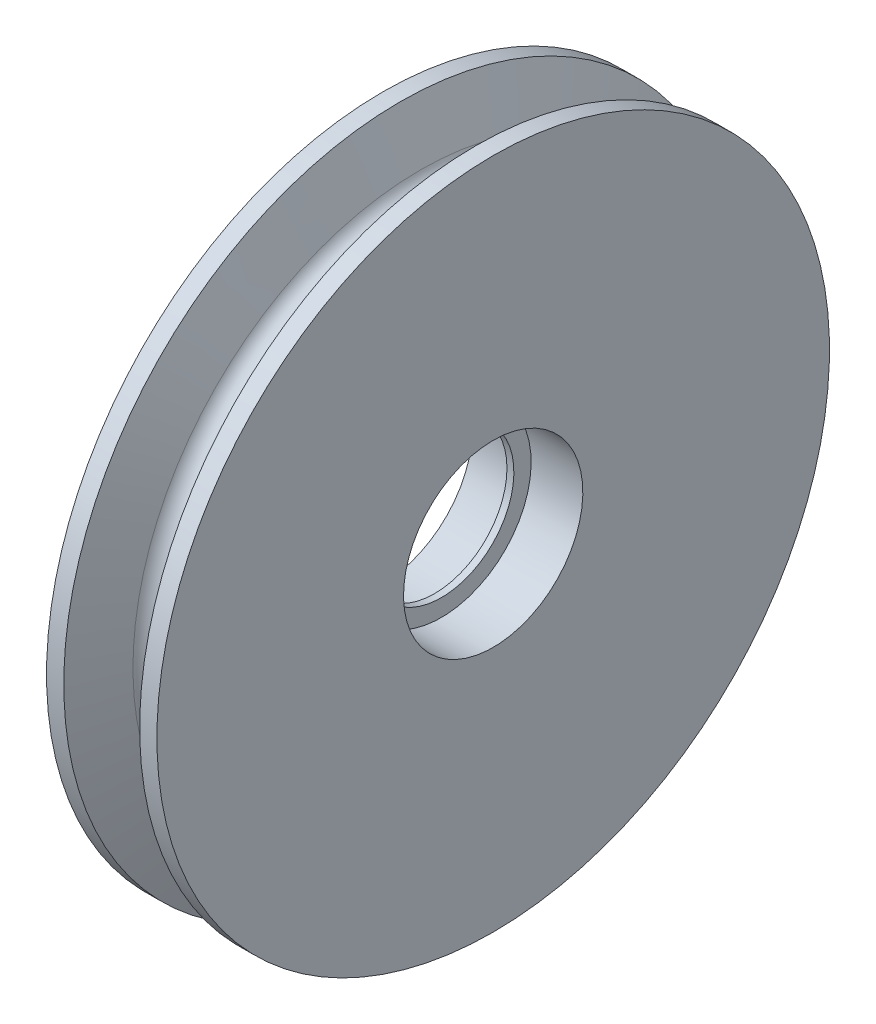
from build123d import *

# Parameters (mm, degrees)
CUT_EXTRUDE1_REACH = 143.55
SKETCH2_R          = 21
SKETCH3_R          = 26
CUT_EXTRUDE2_DEPTH = 15


with BuildPart() as part:
    # Sketch1 → Revolve1 (revolve)
    with BuildSketch(Plane.XY):
        with BuildLine():
            Line((-16, 0), (-16, 97.5))
            Line((-16, 97.5), (-11, 97.5))
            Line((-11, 97.5), (-5.071594443, 83.37187176))
            ThreePointArc((-5.071594443, 83.37187176), (0, 80), (5.071594443, 83.37187176))
            Line((5.071594443, 83.37187176), (11, 97.5))
            Line((11, 97.5), (16, 97.5))
            Line((16, 97.5), (16, 0))
            Line((16, 0), (-16, 0))
        make_face()
    revolve(axis=Axis((16, 0, 0), (-1, 0, 0)))

    # Sketch2 → Cut-Extrude1 (cut, up to next)
    with BuildSketch(Plane(origin=(16, 0, 0), x_dir=(0, 0, -1), z_dir=(1, 0, 0)), mode=Mode.PRIVATE) as cut_extrude1_sk1:
        with Locations(Location((0, 0, 0), (0, 0, 90))):
            Circle(SKETCH2_R)
    cut_extrude1_tool1 = extrude(cut_extrude1_sk1.sketch, amount=-CUT_EXTRUDE1_REACH, mode=Mode.PRIVATE) & part.part
    add(cut_extrude1_tool1.solids().sort_by_distance((16, 0, 0))[0], mode=Mode.SUBTRACT)

    # Sketch3 → Cut-Extrude2 (cut)
    with BuildSketch(Plane(origin=(16, 0, 0), x_dir=(0, 0, -1), z_dir=(1, 0, 0))):
        with Locations(Location((0, 0, 0), (0, 0, 90))):
            Circle(SKETCH3_R)
    cut_extrude2 = extrude(amount=-CUT_EXTRUDE2_DEPTH, mode=Mode.SUBTRACT)

    # Mirror1: Cut-Extrude2 across plane
    add(cut_extrude2.mirror(Plane(origin=(0, 0, 0), x_dir=(0, 0, 1), z_dir=(1, 0, 0))), mode=Mode.SUBTRACT)


solid = part.part
